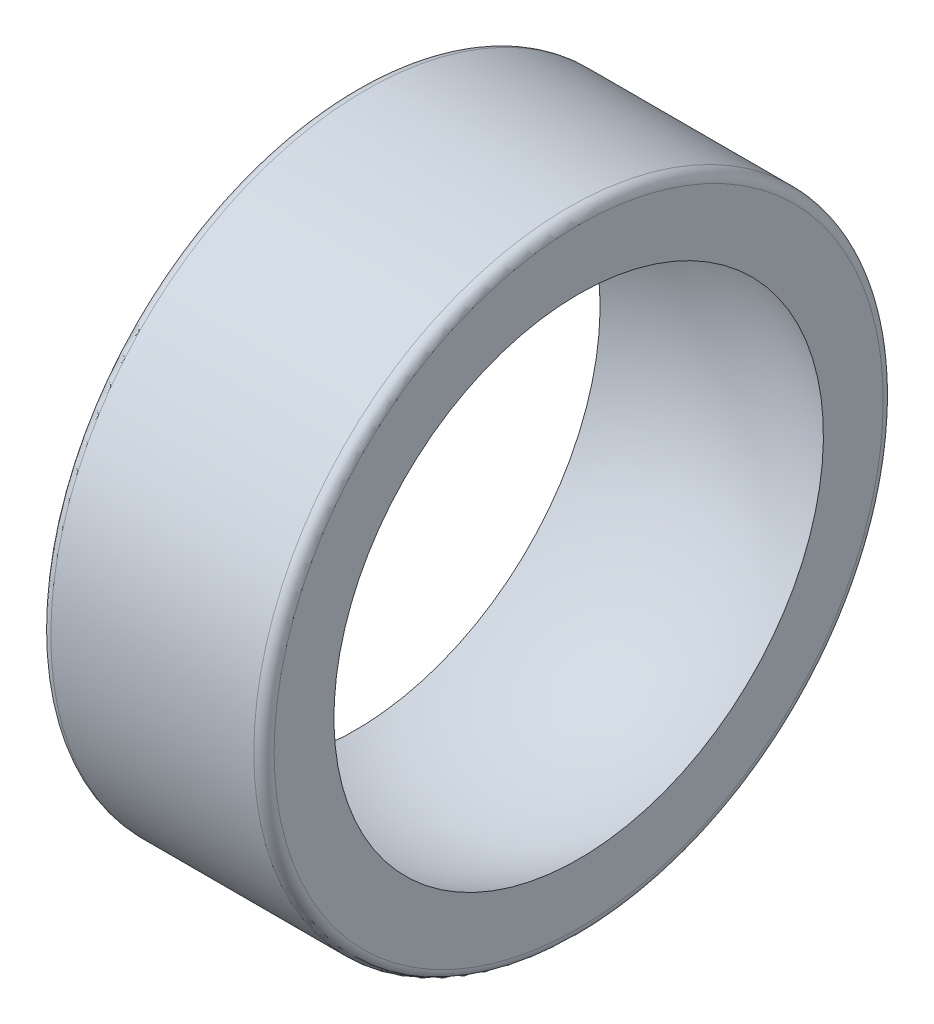
from build123d import *

# Parameters (mm, degrees)
FILLET_1_R = 1


with BuildPart() as part:
    # 草图2 → 旋转1 (revolve)
    with BuildSketch(Plane.XY, mode=Mode.PRIVATE) as revolve_1_sk:
        with BuildLine():
            Line((-11, 31), (-11, 24.109126902))
            ThreePointArc((-11, 24.109126902), (0, 26.5), (11, 24.109126902))
            Line((11, 24.109126902), (11, 31))
            Line((11, 31), (-11, 31))
        make_face()
    revolve(revolve_1_sk.sketch.rotate(Axis((-53.012504143, 0, 0), (1, 0, 0)), 90), axis=Axis((-53.012504143, 0, 0), (1, 0, 0)))

    # 圆角1
    fillet_1_edges = [part.edges().sort_by_distance(p)[0] for p in [
        (11, 0, -31),
        (-11, 0, -31),
    ]]
    fillet(fillet_1_edges, radius=FILLET_1_R)


solid = part.part
